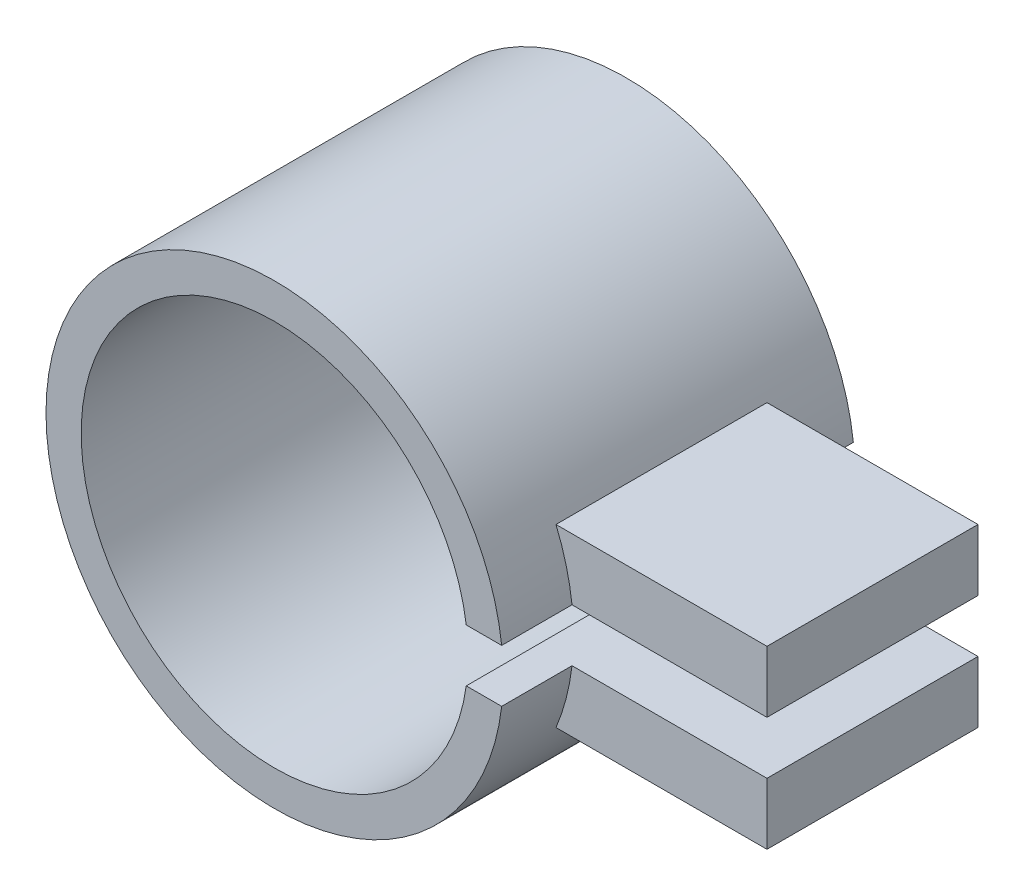
SolidWorks part; units mm, degrees
material "316L"
ref_plane "Front Plane" through (0, 0, 0) normal (0, 0, 1) x (1, 0, 0)
ref_plane "Top Plane" through (0, 0, 0) normal (0, 1, 0) x (1, 0, 0)
ref_plane "Right Plane" through (0, 0, 0) normal (1, 0, 0) x (0, 0, -1)
sketch "Sketch1" plane through (0, 0, 0) normal (0, 0, 1) x (1, 0, 0)
  circle A0 centre (0, 0) radius 5.5
  dimension "D1" = 11
extrude "Extrude-Thin1" add sketch "Sketch1" along normal mid plane 10 thin
sketch "Sketch2" plane through (0, 0, 0) normal (0, 0, 1) x (1, 0, 0)
  line L1 (6, 2.5) -> (12, 2.5)
  line L2 (6, 2.5) -> (6, -2.5)
  line L3 (6, -2.5) -> (12, -2.5)
  line L4 (12, 2.5) -> (12, -2.5)
  circle A0 centre (0, 0) radius 6.5 construction
  dimension "D1" = 5
  dimension "D2" = 6
extrude "Boss-Extrude1" add sketch "Sketch2" along normal mid plane 6
sketch "Sketch4" plane through (0, 0, 5) normal (0, 0, 1) x (1, 0, 0)
  line L1 (0, 0.75) -> (14.2231, 0.75)
  line L2 (0, 0.75) -> (0, -0.75)
  line L3 (0, -0.75) -> (14.2231, -0.75)
  line L4 (14.2231, 0.75) -> (14.2231, -0.75)
  dimension "D1" = 1.5
extrude "Cut-Extrude1" cut sketch "Sketch4" against normal through all
